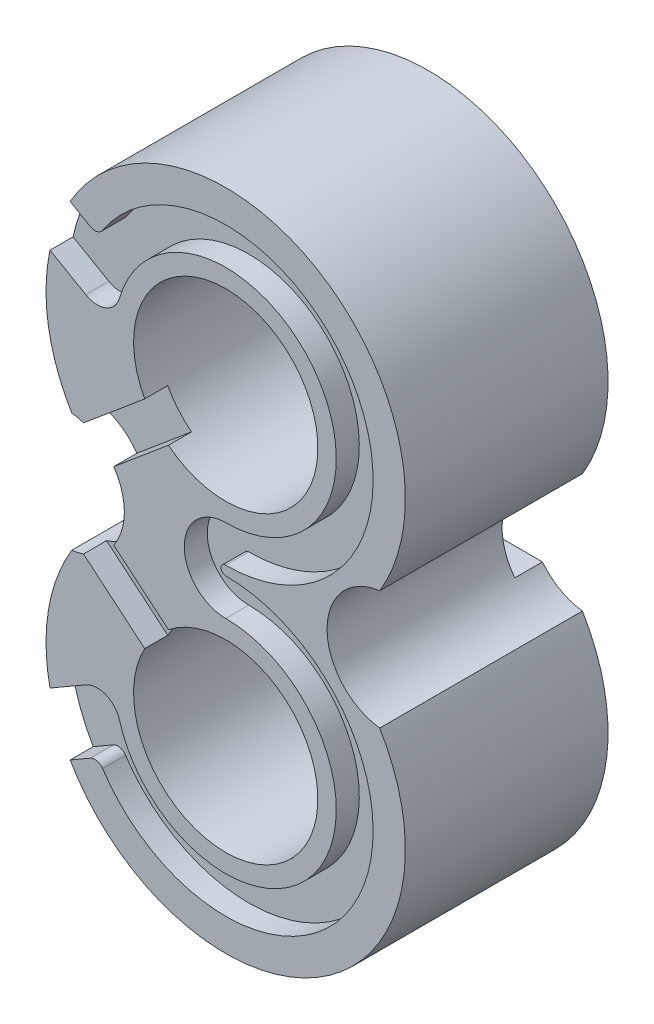
from build123d import *

# Parameters (mm, degrees)
SKETCH1_R           = 10
BOSS_EXTRUDE1_DEPTH = 11
CUT_EXTRUDE1_DEPTH  = 2.5
CUT_EXTRUDE2_DEPTH  = 2.5
SKETCH4_W           = 15.449608091
SKETCH4_H           = 8
CUT_EXTRUDE3_DEPTH  = 3
FILLET1_R           = 1
CUT_EXTRUDE5_START  = -1.5
CUT_EXTRUDE5_DEPTH  = 1.5


with BuildPart() as part:
    # Sketch1 → Boss-Extrude1 (new, symmetric)
    with BuildSketch(Plane.XY):
        with BuildLine():
            ThreePointArc((16.711932938, -6.452050085), (11, 0), (16.711932938, 6.452050085))
            ThreePointArc((16.711932938, 6.452050085), (0, 36), (-16.711932938, 6.452050085))
            ThreePointArc((-16.711932938, 6.452050085), (-11, 0), (-16.711932938, -6.452050085))
            ThreePointArc((-16.711932938, -6.452050085), (0, -36), (16.711932938, -6.452050085))
        make_face()
        with Locations((0, -16.5)):
            Circle(SKETCH1_R, mode=Mode.SUBTRACT)
        with Locations((0, 16.5)):
            Circle(SKETCH1_R, mode=Mode.SUBTRACT)
    extrude(amount=BOSS_EXTRUDE1_DEPTH, both=True)

    # Sketch2 → Cut-Extrude1 (cut)
    with BuildSketch(Plane.XY.offset(11)):
        with BuildLine():
            Line((-19.068213964, 20.580835235), (-15.186057607, 18.339471217))
            ThreePointArc((-15.186057607, 18.339471217), (-13.000189211, 18.186313351), (-11.533289054, 19.814097705))
            ThreePointArc((-11.533289054, 19.814097705), (9.5856448, 23.719100621), (0, 4.5))
            ThreePointArc((0, 4.5), (-4.5, 0), (0, -4.5))
            ThreePointArc((0, -4.5), (9.5856448, -23.719100621), (-11.533289054, -19.814097705))
            ThreePointArc((-11.533289054, -19.814097705), (-13.000189211, -18.186313351), (-15.186057607, -18.339471217))
            Line((-15.186057607, -18.339471217), (-19.068213964, -20.580835235))
            ThreePointArc((-19.068213964, -20.580835235), (-18.199948236, -23.500848821), (-16.887495374, -26.25))
            Line((-16.887495374, -26.25), (-14.696938457, -24.985281374))
            ThreePointArc((-14.696938457, -24.985281374), (-13.966653368, -24.87818357), (-13.36182443, -25.301229909))
            ThreePointArc((-13.36182443, -25.301229909), (14.085802756, -24.088818138), (0, -0.5))
            ThreePointArc((0, -0.5), (-0.5, 0), (0, 0.5))
            ThreePointArc((0, 0.5), (14.085802756, 24.088818138), (-13.36182443, 25.301229909))
            ThreePointArc((-13.36182443, 25.301229909), (-13.966653368, 24.87818357), (-14.696938457, 24.985281374))
            Line((-14.696938457, 24.985281374), (-16.887495374, 26.25))
            ThreePointArc((-16.887495374, 26.25), (-18.199948236, 23.500848821), (-19.068213964, 20.580835235))
        make_face()
    extrude(amount=-CUT_EXTRUDE1_DEPTH, mode=Mode.SUBTRACT)

    # Sketch3 → Cut-Extrude2 (cut)
    with BuildSketch(Plane.XY.offset(11)):
        Polygon((-17.173443463, 0.521044654), (1.285575219, -14.967911114), (-1.285575219, -18.032088886), (-19.744593902, -2.543133118), align=None)
    cut_extrude2 = extrude(amount=-CUT_EXTRUDE2_DEPTH, mode=Mode.SUBTRACT)

    # Mirror1: Cut-Extrude2 across plane
    add(cut_extrude2.mirror(Plane.ZX), mode=Mode.SUBTRACT)

    # Sketch4 → Cut-Extrude3 (cut)
    with BuildSketch(Plane(origin=(0, 0, -11), x_dir=(-1, 0, 0), z_dir=(0, 0, -1))):
        with Locations((11.224804046, 0)):
            Rectangle(SKETCH4_W, SKETCH4_H)
        with Locations((-11.224804046, 0)):
            Rectangle(SKETCH4_W, SKETCH4_H)
    extrude(amount=-CUT_EXTRUDE3_DEPTH, mode=Mode.SUBTRACT)

    # Fillet1
    fillet1_edges = [part.edges().sort_by_distance(p)[0] for p in [
        (-3.5, 4, -9.5),
        (-3.5, -4, -9.5),
        (3.5, -4, -9.5),
        (3.5, 4, -9.5),
    ]]
    fillet(fillet1_edges, radius=FILLET1_R)

    # Sketch5 → Cut-Extrude5 (cut)
    with BuildSketch(Plane(origin=(0, 0, -11), x_dir=(-1, 0, 0), z_dir=(0, 0, -1)).offset(CUT_EXTRUDE5_START)):
        with BuildLine():
            ThreePointArc((12.376524617, 4), (13.243803843, 4.912717605), (14.270776222, 5.641109269))
            Line((14.270776222, 5.641109269), (7.397387325, 9.771057976))
            ThreePointArc((7.397387325, 9.771057976), (5.606135542, 8.219224415), (3.5, 7.132503002))
            Line((3.5, 7.132503002), (3.5, 3))
            ThreePointArc((3.5, 3), (3.792893219, 3.707106781), (4.5, 4))
            Line((4.5, 4), (12.376524617, 4))
        make_face()
        with BuildLine():
            Line((7.397387325, -9.771057976), (14.270776222, -5.641109269))
            ThreePointArc((14.270776222, -5.641109269), (13.243803843, -4.912717605), (12.376524617, -4))
            Line((12.376524617, -4), (4.5, -4))
            ThreePointArc((4.5, -4), (3.792893219, -3.707106781), (3.5, -3))
            Line((3.5, -3), (3.5, -7.132503002))
            ThreePointArc((3.5, -7.132503002), (5.606135542, -8.219224415), (7.397387325, -9.771057976))
        make_face()
    extrude(amount=CUT_EXTRUDE5_DEPTH, mode=Mode.SUBTRACT)


solid = part.part
